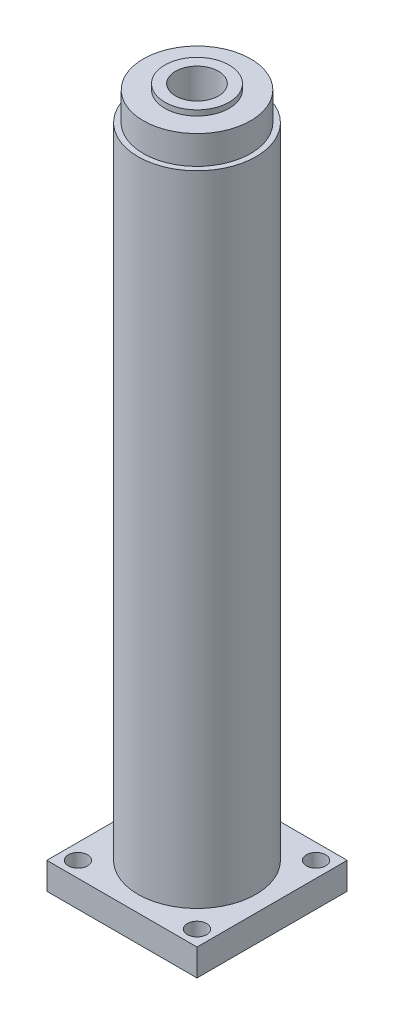
from build123d import *

# Parameters (mm, degrees)
SKETCH1_W           = 140
SKETCH1_H           = 140
SKETCH1_R           = 9
BOSS_EXTRUDE1_DEPTH = 25
SKETCH2_R           = 55
BOSS_EXTRUDE2_DEPTH = 652
SKETCH3_R           = 20
CUT_EXTRUDE1_DEPTH  = 1580
SKETCH4_OUTSIDE_W   = 278.28
SKETCH4_OUTSIDE_H   = 278.28
SKETCH4_OUTSIDE_R   = 30
CUT_EXTRUDE2_DEPTH  = 5
SKETCH6_OUTSIDE_W   = 278.28
SKETCH6_OUTSIDE_H   = 278.28
SKETCH6_OUTSIDE_R   = 50
CUT_EXTRUDE3_DEPTH  = 31.5


with BuildPart() as part:
    # Sketch1 → Boss-Extrude1 (new body)
    with BuildSketch(Plane(origin=(0, 0, 0), x_dir=(1, 0, 0), z_dir=(0, 1, 0))):
        Rectangle(SKETCH1_W, SKETCH1_H)
        with Locations(Location((-55.5, 55.5, 0), (0, 0, 270))):
            Circle(SKETCH1_R, mode=Mode.SUBTRACT)
        with Locations(Location((55.5, 55.5, 0), (0, 0, 270))):
            Circle(SKETCH1_R, mode=Mode.SUBTRACT)
        with Locations(Location((55.5, -55.5, 0), (0, 0, 270))):
            Circle(SKETCH1_R, mode=Mode.SUBTRACT)
        with Locations(Location((-55.5, -55.5, 0), (0, 0, 270))):
            Circle(SKETCH1_R, mode=Mode.SUBTRACT)
    extrude(amount=BOSS_EXTRUDE1_DEPTH)

    # Sketch2 → Boss-Extrude2 (add)
    with BuildSketch(Plane(origin=(0, 0, 0), x_dir=(1, 0, 0), z_dir=(0, 1, 0))):
        with Locations(Location((0, 0, 0), (0, 0, 270))):
            Circle(SKETCH2_R)
    extrude(amount=BOSS_EXTRUDE2_DEPTH)

    # Sketch3 → Cut-Extrude1 (cut)
    with BuildSketch(Plane(origin=(0, 652, 0), x_dir=(1, 0, 0), z_dir=(0, 1, 0))):
        with Locations(Location((0, 0, 0), (0, 0, 270))):
            Circle(SKETCH3_R)
    extrude(amount=-CUT_EXTRUDE1_DEPTH, mode=Mode.SUBTRACT)

    # Sketch4 outside → Cut-Extrude2 (cut)
    with BuildSketch(Plane(origin=(0, 652, 0), x_dir=(1, 0, 0), z_dir=(0, 1, 0))):
        Rectangle(SKETCH4_OUTSIDE_W, SKETCH4_OUTSIDE_H)
        with Locations(Location((0, 0, 0), (0, 0, 270))):
            Circle(SKETCH4_OUTSIDE_R, mode=Mode.SUBTRACT)
    extrude(amount=-CUT_EXTRUDE2_DEPTH, mode=Mode.SUBTRACT)

    # Sketch6 outside → Cut-Extrude3 (cut)
    with BuildSketch(Plane(origin=(0, 652, 0), x_dir=(1, 0, 0), z_dir=(0, 1, 0))):
        Rectangle(SKETCH6_OUTSIDE_W, SKETCH6_OUTSIDE_H)
        with Locations(Location((0, 0, 0), (0, 0, 270))):
            Circle(SKETCH6_OUTSIDE_R, mode=Mode.SUBTRACT)
    extrude(amount=-CUT_EXTRUDE3_DEPTH, mode=Mode.SUBTRACT)


solid = part.part
